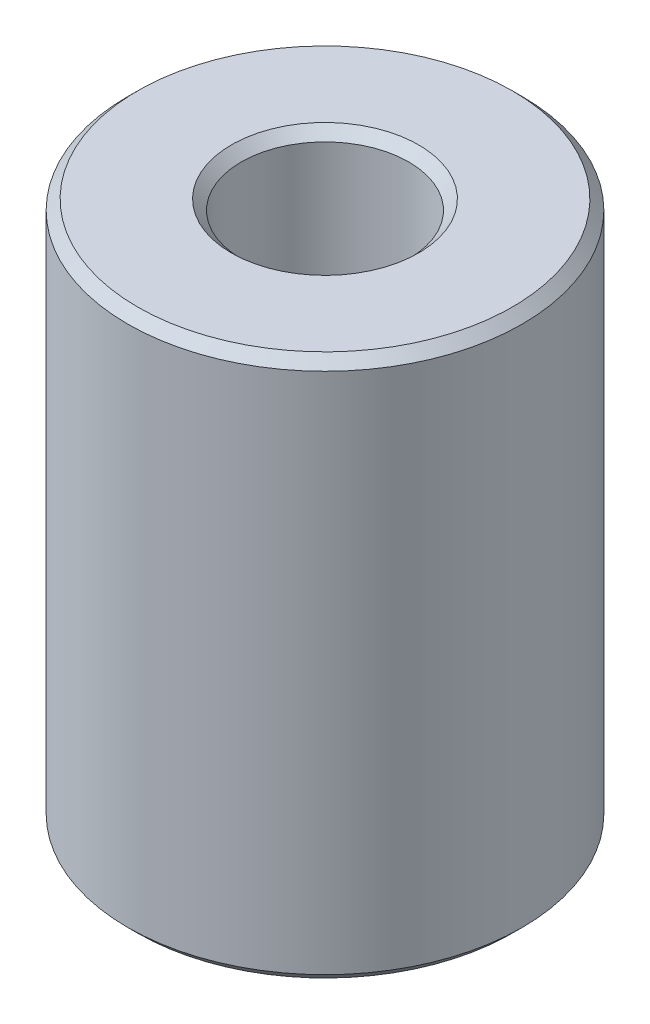
from build123d import *

# Parameters (mm, degrees)
SKETCH_1_R          = 20
EXTRUDE_1_DEPTH     = 55
SKETCH_2_R          = 8.5
CUT_EXTRUDE_1_DEPTH = 20
SKETCH_3_R          = 10
CUT_EXTRUDE_2_DEPTH = 20
CHAMFER_1_SIZE      = 1


with BuildPart() as part:
    # 草图1 → 凸台-拉伸1 (new body)
    with BuildSketch(Plane(origin=(0, 0, 0), x_dir=(1, 0, 0), z_dir=(0, 1, 0))):
        with Locations(Location((0, 0, 0), (0, 0, 270))):
            Circle(SKETCH_1_R)
    extrude(amount=EXTRUDE_1_DEPTH)

    # 草图2 → 切除-拉伸1 (cut)
    with BuildSketch(Plane(origin=(0, 55, 0), x_dir=(1, 0, 0), z_dir=(0, 1, 0))):
        with Locations(Location((0, 0, 0), (0, 0, 270))):
            Circle(SKETCH_2_R)
    extrude(amount=-CUT_EXTRUDE_1_DEPTH, mode=Mode.SUBTRACT)

    # 草图3 → 切除-拉伸2 (cut)
    with BuildSketch(Plane.XZ):
        with Locations(Location((0, 0, 0), (0, 0, 270))):
            Circle(SKETCH_3_R)
    extrude(amount=-CUT_EXTRUDE_2_DEPTH, mode=Mode.SUBTRACT)

    # 倒角1
    chamfer_1_edges = [part.edges().sort_by_distance(p)[0] for p in [
        (0, 0, 10),
        (0, 0, -20),
        (0, 55, -20),
        (0, 55, -8.5),
    ]]
    chamfer(chamfer_1_edges, length=CHAMFER_1_SIZE)


solid = part.part
